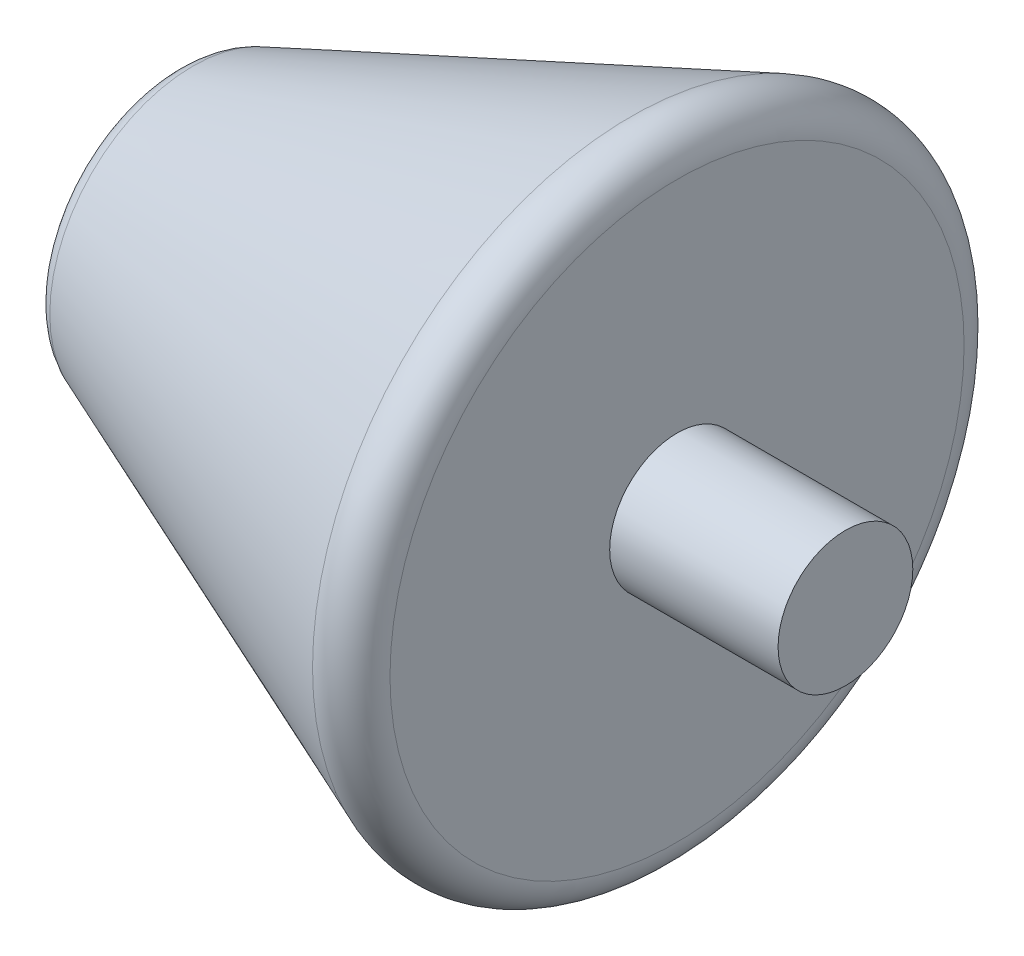
SolidWorks part; units mm, degrees
ref_plane "Front Plane" through (0, 0, 0) normal (0, 0, 1) x (1, 0, 0)
ref_plane "Top Plane" through (0, 0, 0) normal (0, 1, 0) x (1, 0, 0)
ref_plane "Right Plane" through (0, 0, 0) normal (1, 0, 0) x (0, 0, -1)
sketch "Sketch1" plane through (0, 0, 0) normal (0, 0, 1) x (1, 0, 0)
  line L0 (30, 20) -> (30, 0)
  line L1 (0, 0) -> (0, 8)
  line L2 (10.6577, 0) -> (37.5075, 0) construction
  line L3 (0, -55) -> (0, 55) construction
  line L7 (0, 8) -> (30, 20)
  line L8 (0, 0) -> (30, 0)
  dimension "D1" = 30
  dimension "D2" = 20
revolve "Revolve1" add sketch "Sketch1" angle 360 about L2
fillet "Fillet1" radius 2 1 edges at (0, 0, 8)
sketch "Sketch2" plane through (30, 0, 0) normal (1, 0, 0) x (0, 0, -1)
  circle A0 centre (0, 0) radius 4
  dimension "D1" = 8
extrude "Boss-Extrude1" add sketch "Sketch2" along normal blind 10
fillet "Fillet2" radius 2 1 edges at (30, 0, 20)
